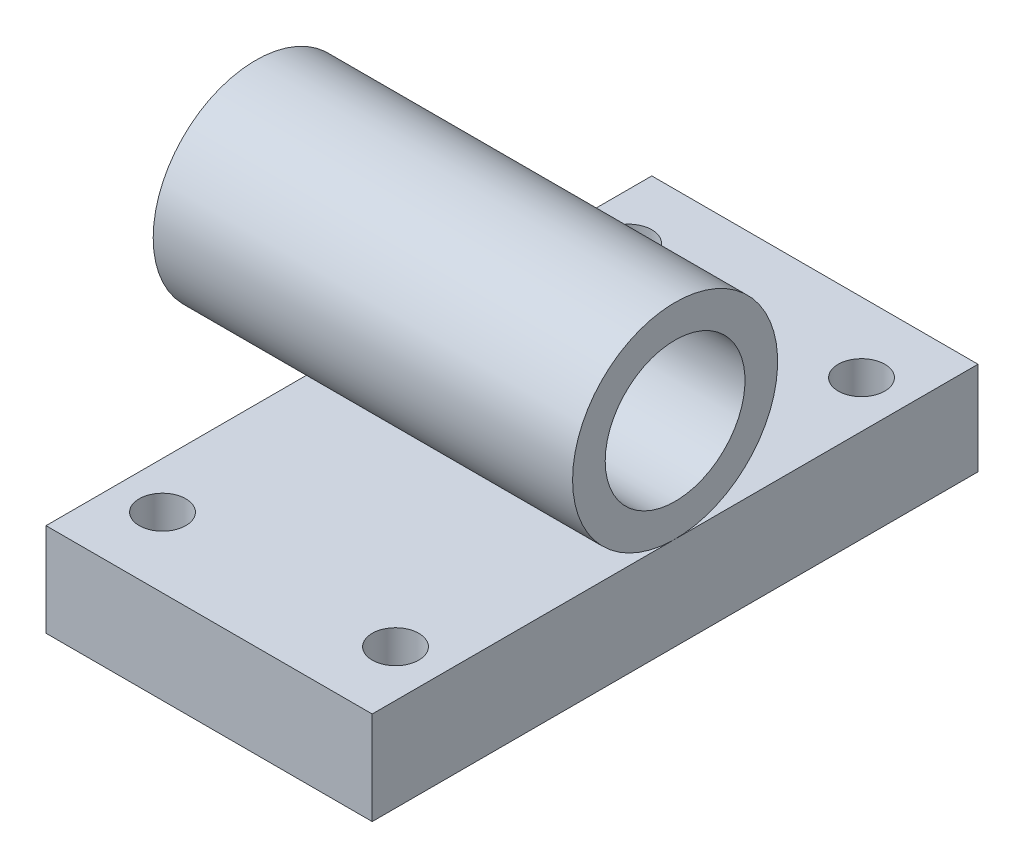
from build123d import *

# Parameters (mm, degrees)
SKETCH_1_W      = 70
SKETCH_1_H      = 130
SKETCH_1_R      = 5
EXTRUDE_1_DEPTH = 20
SKETCH_4_W      = 3.4
SKETCH_4_H      = 65


with BuildPart() as part:
    # 草图1 → 凸台-拉伸1 (new body)
    with BuildSketch(Plane(origin=(0, 0, 0), x_dir=(1, 0, 0), z_dir=(0, 1, 0))):
        Rectangle(SKETCH_1_W, SKETCH_1_H)
        with Locations(Location((-25, -50, 0), (0, 0, 270))):
            Circle(SKETCH_1_R, mode=Mode.SUBTRACT)
        with Locations(Location((25, -50, 0), (0, 0, 270))):
            Circle(SKETCH_1_R, mode=Mode.SUBTRACT)
        with Locations(Location((25, 50, 0), (0, 0, 270))):
            Circle(SKETCH_1_R, mode=Mode.SUBTRACT)
        with Locations(Location((-25, 50, 0), (0, 0, 270))):
            Circle(SKETCH_1_R, mode=Mode.SUBTRACT)
    extrude(amount=EXTRUDE_1_DEPTH)


with BuildPart() as body_2:
    # 草图2 → 旋转1 (revolve)
    with BuildSketch(Plane.XY, mode=Mode.PRIVATE) as revolve_1_sk:
        Polygon((-55, 50), (-47, 50), (-47, 57), (35, 57), (35, 64), (-55, 64), align=None)
    revolve(revolve_1_sk.sketch.rotate(Axis((-55, 42, 0), (1, 0, 0)), 90), axis=Axis((-55, 42, 0), (1, 0, 0)))

    # 草图4 → M8 螺纹孔1 (revolve, cut)
    with BuildSketch(Plane(origin=(15, 42, 0), x_dir=(0, -1, 0), z_dir=(1, 0, 0))):
        with Locations((1.7, 32.5)):
            Rectangle(SKETCH_4_W, SKETCH_4_H)
    revolve(axis=Axis((15, 42, 6.35), (0, 0, -1)), mode=Mode.SUBTRACT)


solid = Compound([part.part, body_2.part])
